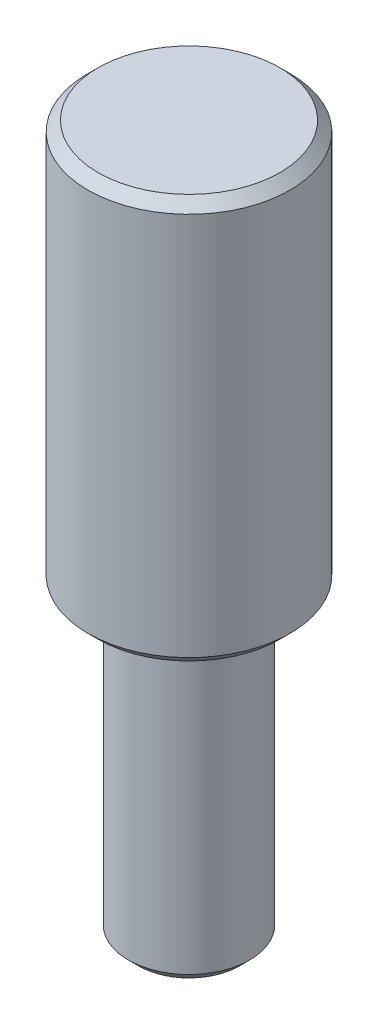
from build123d import *

# Parameters (mm, degrees)
SKETCH1_R           = 5
BOSS_EXTRUDE1_DEPTH = 20
SKETCH2_R           = 3
BOSS_EXTRUDE2_DEPTH = 15
CHAMFER1_SIZE       = 0.5


with BuildPart() as part:
    # Sketch1 → Boss-Extrude1 (new body)
    with BuildSketch(Plane(origin=(0, 0, 0), x_dir=(1, 0, 0), z_dir=(0, 1, 0))):
        with Locations(Location((0, 0, 0), (0, 0, 270))):
            Circle(SKETCH1_R)
    extrude(amount=BOSS_EXTRUDE1_DEPTH)

    # Sketch2 → Boss-Extrude2 (add)
    with BuildSketch(Plane.XZ):
        with Locations(Location((0, 0, 0), (0, 0, 270))):
            Circle(SKETCH2_R)
    extrude(amount=BOSS_EXTRUDE2_DEPTH)

    # Chamfer1
    chamfer1_edges = [part.edges().sort_by_distance(p)[0] for p in [
        (0, 0, -5),
        (0, 20, -5),
        (0, -15, 3),
    ]]
    chamfer(chamfer1_edges, length=CHAMFER1_SIZE)


solid = part.part
